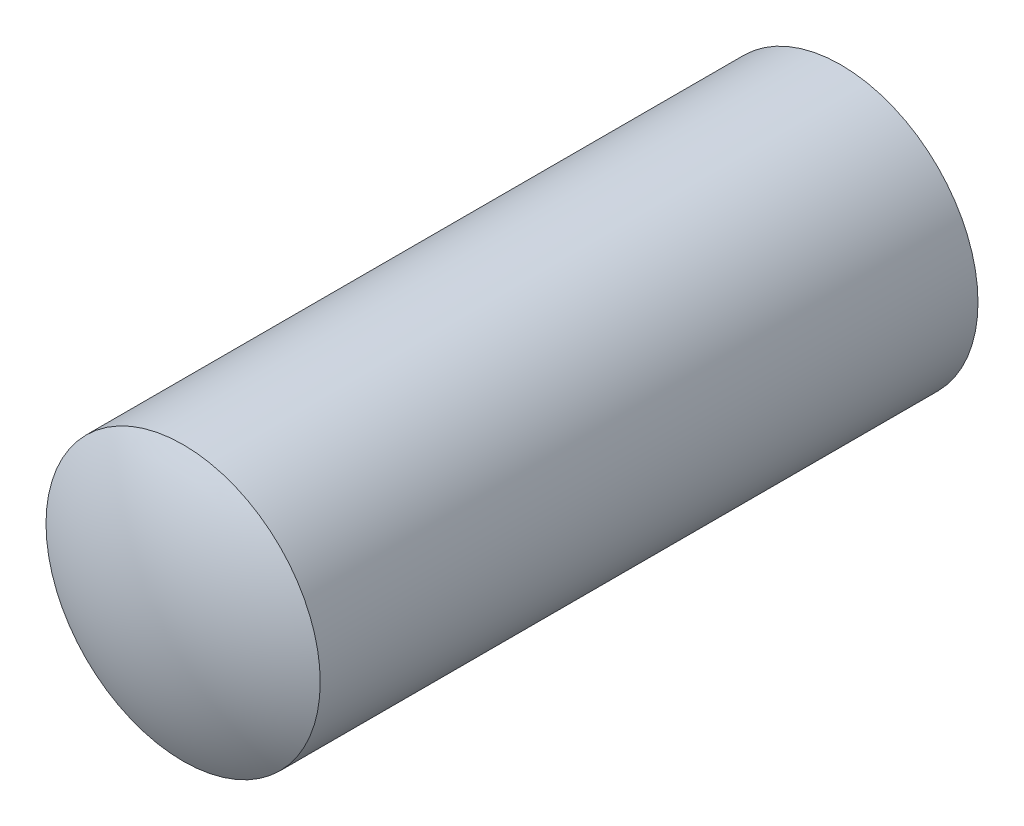
SolidWorks part; units mm, degrees
ref_plane "Front" through (0, 0, 0) normal (0, 0, 1) x (1, 0, 0)
ref_plane "Top" through (0, 0, 0) normal (0, 1, 0) x (1, 0, 0)
ref_plane "Right" through (0, 0, 0) normal (1, 0, 0) x (0, 0, -1)
sketch "Logo3_Revol_Axis" plane through (0, 0, 0) normal (0, 1, 0) x (1, 0, 0)
  line L0 (0, -30.1653) -> (0, 30.1653) construction
sketch "Logo3_bib1" plane through (0, 0, 0) normal (0, -1, 0) x (-1, 0, 0)
  line L0 (0, 6) -> (0, -2)
  line L1 (1.5, 5.5981) -> (1.5, -1.5981)
  line L10 (0, 47.5372) -> (0, -34.1764) construction
  arc A0 (1.5, 5.5981) -> (0, 6) centre (0, 3) ccw
  arc A1 (0, -2) -> (1.5, -1.5981) centre (0, 1) ccw
revolve "Revolve1" add sketch "Logo3_bib1" angle 360 about L10
equation "\"ray2@XZQB7_bib1\" = \"XZQB7_d1@XZQB7_bib1\""
equation "\"Ray1@XZQB7_bib1\" = \"XZQB7_d1@XZQB7_bib1\""
equation "\"dia1@XZQB7_bib1\" = \"XZQB7_d1@XZQB7_bib1\"/2"
